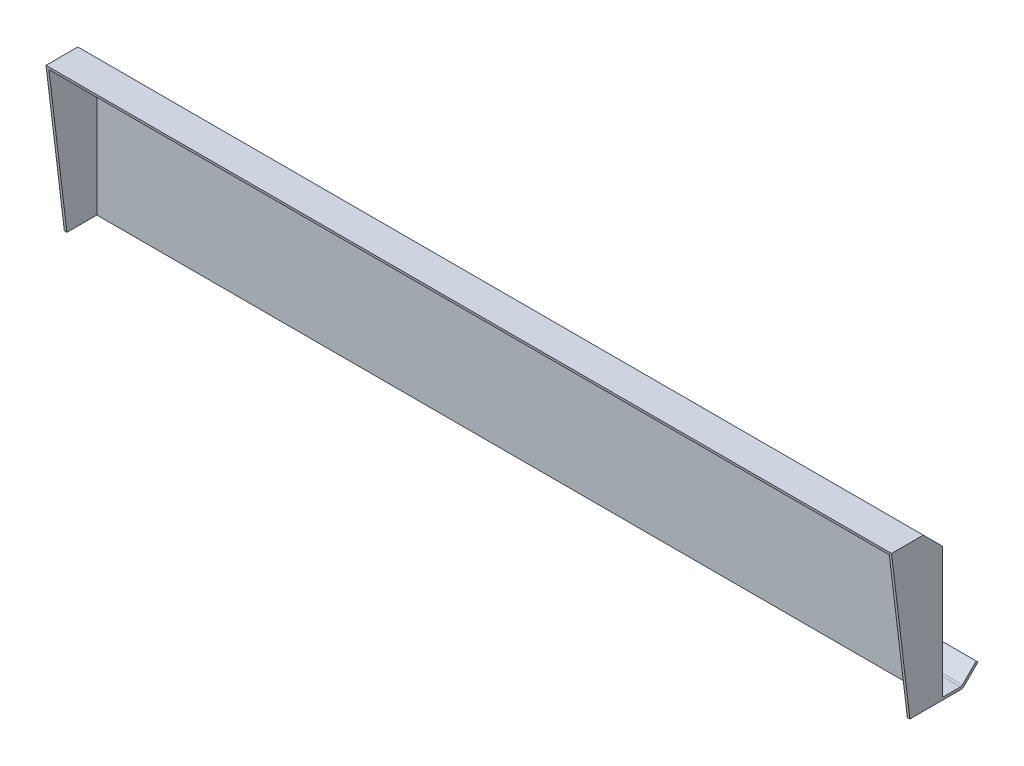
SolidWorks part; units mm, degrees
ref_plane "Front plane" through (0, 0, 0) normal (0, 0, 1) x (1, 0, 0)
ref_plane "Top plane" through (0, 0, 0) normal (0, 1, 0) x (1, 0, 0)
ref_plane "Right plane" through (0, 0, 0) normal (1, 0, 0) x (0, 0, -1)
sketch "Sketch1" plane through (0, 0, 0) normal (1, 0, 0) x (0, 0, -1)
  line L0 (0, 0) -> (40, 0)
  line L5 (14.4466, -120) -> (40, -120)
  line L6 (40, 0) -> (40, -120)
  line L9 (14.4466, -120) -> (0, 0)
  dimension "D3" = 40
  dimension "D1" = 120
  dimension "D2" = 96.865
extrude "Boss-Extrude1" add sketch "Sketch1" along normal mid plane 665
chamfer "Chamfer1" distance 15 angle 45 1 edges at (0, 0, -40)
shell "Shell1" thickness 2
sketch "Sketch7" plane through (0, -118, 0) normal (0, 1, 0) x (1, 0, 0)
  line L4 (-330.5, 38) -> (-330.5, 14.2058)
  line L5 (-330.5, 14.2058) -> (330.5, 14.2058)
  line L6 (330.5, 14.2058) -> (330.5, 38)
  line L7 (330.5, 38) -> (-330.5, 38)
  line L8 (-330.5, 38) -> (-330.5, 14.2058)
  line L9 (-330.5, 14.2058) -> (330.5, 14.2058)
  line L10 (330.5, 14.2058) -> (330.5, 38)
  line L11 (330.5, 38) -> (-330.5, 38)
  dimension "D1" = 0
extrude "Cut-Extrude1" cut sketch "Sketch7" against normal through all
sketch "Sketch8" plane through (332.5, 0, 0) normal (1, 0, 0) x (0, 0, -1)
  line L0 (40, -120) -> (55.1716, -120)
  line L1 (56.5858, -119.4142) -> (68.0208, -107.9792)
  line L2 (68.0208, -107.9792) -> (66.6066, -106.565)
  line L3 (66.6066, -106.565) -> (55.7574, -117.4142)
  line L4 (54.3431, -118) -> (40, -118)
  line L5 (40, -120) -> (40, -15) construction
  line L6 (40, -118) -> (40, -120)
  arc A0 (55.7574, -117.4142) -> (54.3431, -118) centre (54.3431, -116) cw
  arc A1 (56.5858, -119.4142) -> (55.1716, -120) centre (55.1716, -118) cw
  point P13 (56, -120)
  dimension "D6" = 2
  dimension "D1" = 2
  dimension "D2" = 16
  dimension "D3" = 2
  dimension "D4" = 135
  dimension "D5" = 17
extrude "Boss-Extrude2" add sketch "Sketch8" against normal up to surface (665 mm away) up to face at (-332.5, -51, -23.8893)
